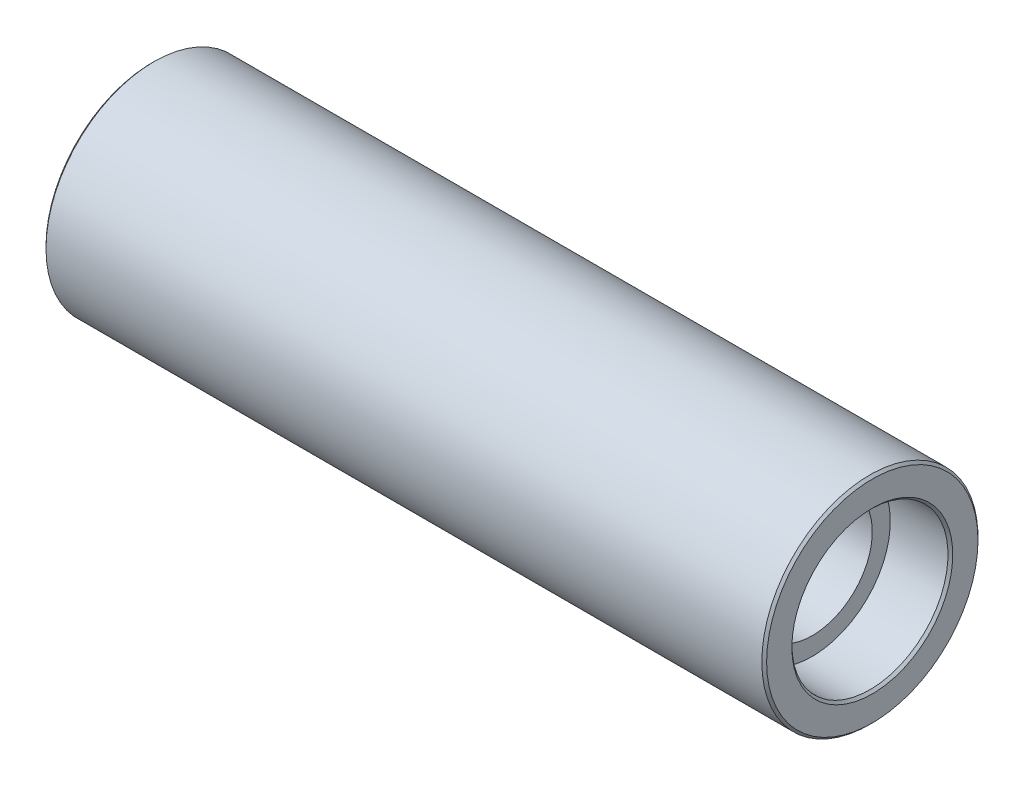
from build123d import *

# Parameters (mm, degrees)
CHAMFER1_SIZE = 0.2


with BuildPart() as part:
    # Sketch1 → Revolve1 (revolve)
    with BuildSketch(Plane.XY, mode=Mode.PRIVATE) as revolve1_sk:
        Polygon((0, 9), (60, 9), (60, 6.5), (55, 6.5), (55, 5), (5, 5), (5, 6.5), (0, 6.5), align=None)
    revolve(revolve1_sk.sketch.rotate(Axis((0, 0, 0), (1, 0, 0)), 90), axis=Axis((0, 0, 0), (1, 0, 0)))

    # Chamfer1
    chamfer1_edges = [part.edges().sort_by_distance(p)[0] for p in [
        (0, 0, -6.5),
        (60, 0, -6.5),
        (60, 0, -9),
        (0, 0, -9),
    ]]
    chamfer(chamfer1_edges, length=CHAMFER1_SIZE)


solid = part.part
